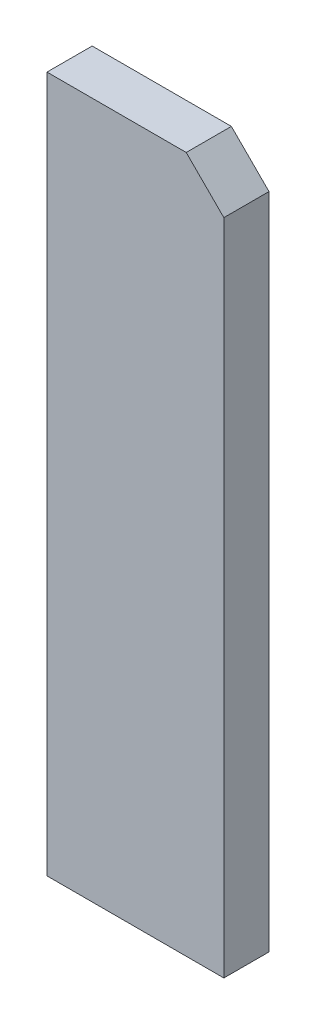
from build123d import *

# Parameters (mm, degrees)
SKETCH_1_W      = 47
SKETCH_1_H      = 185
EXTRUDE_1_DEPTH = 6
CHAMFER_1_SIZE  = 10


with BuildPart() as part:
    # 草图1 → 凸台-拉伸1 (new, symmetric)
    with BuildSketch(Plane.XY):
        with Locations((23.5, 92.5)):
            Rectangle(SKETCH_1_W, SKETCH_1_H)
    extrude(amount=EXTRUDE_1_DEPTH, both=True)

    # 倒角1
    chamfer_1_edges = [part.edges().sort_by_distance(p)[0] for p in [
        (47, 185, 0),
    ]]
    chamfer(chamfer_1_edges, length=CHAMFER_1_SIZE)


solid = part.part
